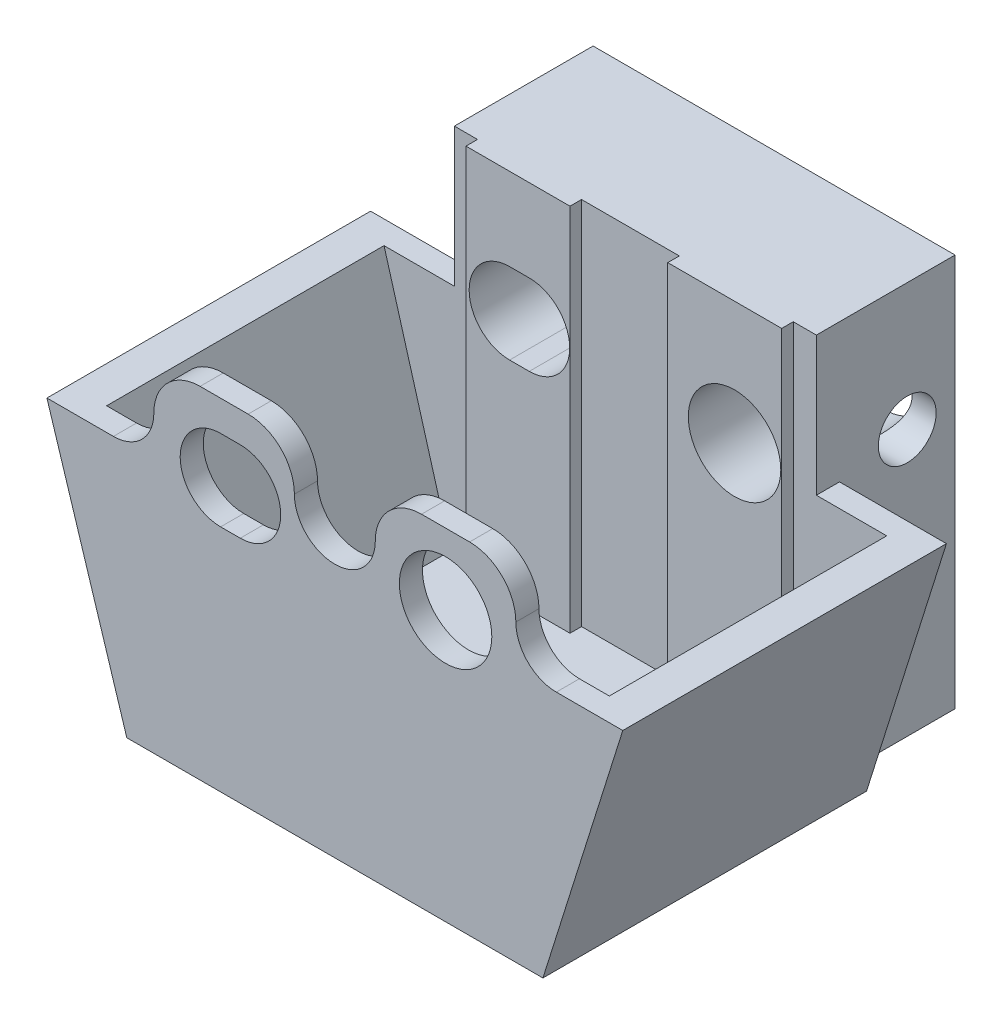
from build123d import *

# Parameters (mm, degrees)
EXTRUDE_2_DEPTH          = 140
EXTRUDE_3_DEPTH          = 140
SKETCH_8_W               = 100
SKETCH_8_H               = 240
CUT_EXTRUDE_1_DEPTH      = 275
EXTRUDE_4_DEPTH          = 100
EXTRUDE_4_DEPTH_BACK     = 20
SKETCH_12_W              = 313.16541006
SKETCH_12_H              = 120
SKETCH_13_W              = 313.16541006
SKETCH_13_H              = 220
EXTRUDE_5_DEPTH          = 100
SKETCH_14_R              = 25
CUT_EXTRUDE_2_DEPTH      = 582.186358517
SKETCH_15_W              = 90
SKETCH_15_H              = 10
SKETCH_15_W_2            = 98.58270503
EXTRUDE_6_DEPTH          = 320
CUT_EXTRUDE_3_DEPTH      = 615.919414052
CUT_EXTRUDE_3_DEPTH_BACK = 615.919414052
SKETCH_16_R              = 40


with BuildPart() as part:
    # 草图1 → 凸台-拉伸2 (new body)
    with BuildSketch(Plane.XY):
        with BuildLine():
            Line((0, 0), (180, 0))
            Line((180, 0), (180, 220))
            ThreePointArc((180, 220), (155.251262658, 230.251262658), (145, 255))
            ThreePointArc((145, 255), (133.284271247, 283.284271247), (105, 295))
            Line((105, 295), (63.41729497, 295))
            ThreePointArc((63.41729497, 295), (35.133023723, 283.284271247), (23.41729497, 255))
            ThreePointArc((23.41729497, 255), (13.166032312, 230.251262658), (-11.58270503, 220))
            Line((-11.58270503, 220), (-69.098922823, 220))
            Line((-69.098922823, 220), (0, 0))
        make_face()
    extrude_2 = extrude(amount=EXTRUDE_2_DEPTH)

    # 草图5 → 凸台-拉伸3 (add)
    with BuildSketch(Plane(origin=(0, 0, 0), x_dir=(-1, 0, 0), z_dir=(0, 0, -1))):
        Polygon((-180, 220), (69.098922823, 220), (0, 0), (-180, 0), align=None)
    extrude_3 = extrude(amount=EXTRUDE_3_DEPTH)

    # 草图8 → 切除-拉伸1 (cut)
    with BuildSketch(Plane(origin=(0, 295, 0), x_dir=(1, 0, 0), z_dir=(0, 1, 0))):
        with Locations((130, 0)):
            Rectangle(SKETCH_8_W, SKETCH_8_H)
    cut_extrude_1 = extrude(amount=-CUT_EXTRUDE_1_DEPTH, mode=Mode.SUBTRACT)

    # 草图10 → 切除-放样4 section 0
    with BuildSketch(Plane(origin=(0, 20, 0), x_dir=(1, 0, 0), z_dir=(0, 1, 0))):
        with BuildLine():
            Line((80, 120), (20, 120))
            Line((20, 120), (20, -120))
            Line((20, -120), (80, -120))
            Line((80, -120), (80, 120))
        make_face()
    # 草图11 → 切除-放样4 section 1
    with BuildSketch(Plane(origin=(0, 295, 0), x_dir=(1, 0, 0), z_dir=(0, 1, 0))):
        with BuildLine():
            Line((80, 120), (80, -120))
            Line((80, -120), (-59, -120))
            Line((-59, -120), (-59, 120))
            Line((-59, 120), (80, 120))
        make_face()
    loft_4 = loft(mode=Mode.SUBTRACT)

    # 镜向1: 凸台-拉伸2, 凸台-拉伸3, 切除-拉伸1, 切除-放样4 across plane
    add(extrude_2.mirror(Plane(origin=(180, 0, 140), x_dir=(0, 0, 1), z_dir=(-1, 0, 0))))
    add(extrude_3.mirror(Plane(origin=(180, 0, 140), x_dir=(0, 0, 1), z_dir=(-1, 0, 0))))
    add(cut_extrude_1.mirror(Plane(origin=(180, 0, 140), x_dir=(0, 0, 1), z_dir=(-1, 0, 0))), mode=Mode.SUBTRACT)
    add(loft_4.mirror(Plane(origin=(180, 0, 140), x_dir=(0, 0, 1), z_dir=(-1, 0, 0))), mode=Mode.SUBTRACT)

    # 草图12 → 凸台-拉伸4 (add, two sides: drawn at the far end of the back side and taken through both)
    with BuildSketch(Plane(origin=(0, 0, -140), x_dir=(-1, 0, 0), z_dir=(0, 0, -1)).offset(-EXTRUDE_4_DEPTH_BACK)):
        with Locations((-180, 280)):
            Rectangle(SKETCH_12_W, SKETCH_12_H)
    extrude(amount=EXTRUDE_4_DEPTH + EXTRUDE_4_DEPTH_BACK)

    # 草图13 → 凸台-拉伸5 (add)
    with BuildSketch(Plane(origin=(0, 0, -140), x_dir=(-1, 0, 0), z_dir=(0, 0, -1))):
        with Locations((-180, 110)):
            Rectangle(SKETCH_13_W, SKETCH_13_H)
    extrude(amount=EXTRUDE_5_DEPTH)

    # 草图14 → 切除-拉伸2 (cut, through all)
    with BuildSketch(Plane(origin=(336.58270503, 0, 0), x_dir=(0, 0, -1), z_dir=(1, 0, 0))):
        with Locations(Location((198.620904307, 230, 0), (0, 0, 90))):
            Circle(SKETCH_14_R)
    extrude(amount=-CUT_EXTRUDE_2_DEPTH, mode=Mode.SUBTRACT)

    # 草图15 → 凸台-拉伸6 (add)
    with BuildSketch(Plane(origin=(0, 340, 0), x_dir=(1, 0, 0), z_dir=(0, 1, 0))):
        with Locations((88.41729497, 115)):
            Rectangle(SKETCH_15_W, SKETCH_15_H)
        with Locations((267.291352515, 115)):
            Rectangle(SKETCH_15_W_2, SKETCH_15_H)
    extrude(amount=-EXTRUDE_6_DEPTH)

    # 草图16 → 切除-拉伸3 (cut, two sides: drawn at the far end of the back side and taken through both)
    with BuildSketch(Plane(origin=(0, 0, -140), x_dir=(-1, 0, 0), z_dir=(0, 0, -1)).offset(-CUT_EXTRUDE_3_DEPTH_BACK)):
        with Locations(Location((-275.791352515, 233.606267036, 0), (0, 0, 90))):
            Circle(SKETCH_16_R)
        with BuildLine():
            Line((-98.176420136, 268.606267036), (-81.17642014, 268.606267036))
            ThreePointArc((-81.17642014, 268.606267036), (-46.17642014, 233.606267036), (-81.17642014, 198.606267036))
            Line((-81.17642014, 198.606267036), (-98.176420136, 198.606267036))
            ThreePointArc((-98.176420136, 198.606267036), (-133.176420136, 233.606267036), (-98.176420136, 268.606267036))
        make_face()
    extrude(amount=CUT_EXTRUDE_3_DEPTH + CUT_EXTRUDE_3_DEPTH_BACK, mode=Mode.SUBTRACT)


solid = part.part
